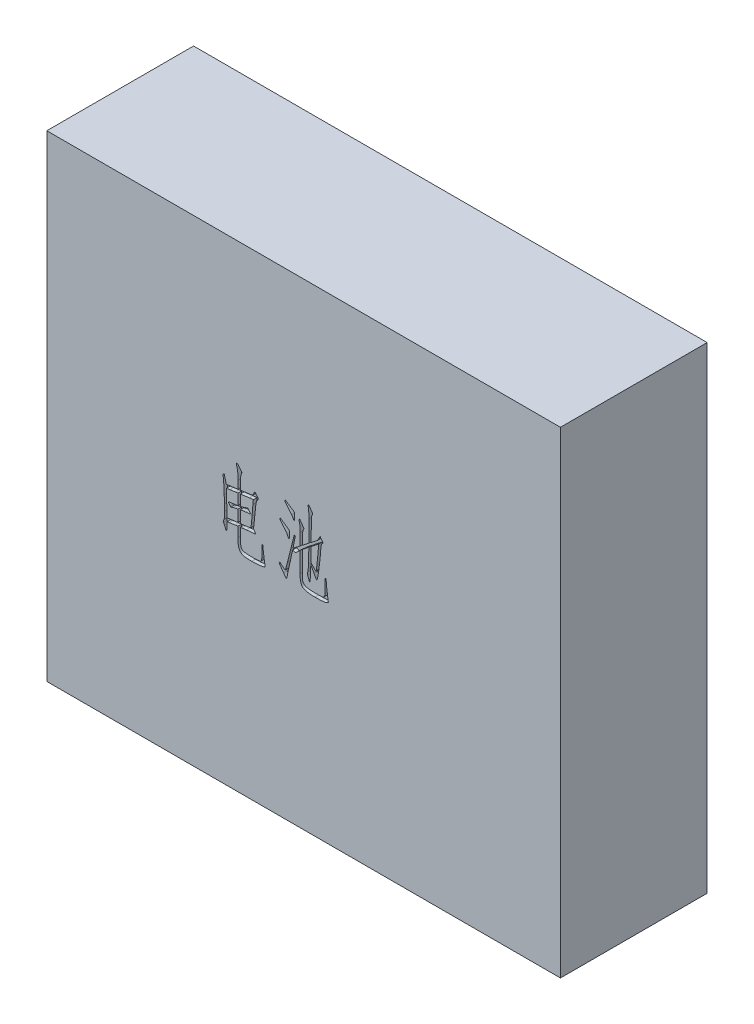
SolidWorks part; units mm, degrees
ref_plane "Front Plane" through (0, 0, 0) normal (0, 0, 1) x (1, 0, 0)
ref_plane "Top Plane" through (0, 0, 0) normal (0, 1, 0) x (1, 0, 0)
ref_plane "Right Plane" through (0, 0, 0) normal (1, 0, 0) x (0, 0, -1)
other "Configuration Table"
sketch "Sketch1" plane through (0, 0, 0) normal (0, 0, 1) x (1, 0, 0)
  line L1 (0, 0) -> (-70, 0)
  line L2 (0, 0) -> (0, 65)
  line L3 (0, 65) -> (-70, 65)
  line L4 (-70, 0) -> (-70, 65)
  dimension "D1" = 70
  dimension "D2" = 65
extrude "Boss-Extrude1" add sketch "Sketch1" along normal blind 20
sketch "Sketch2" plane through (0, 0, 20) normal (0, 0, 1) x (1, 0, 0)
  line L0 (-47.4818, 29.6161) -> (-11.9284, 29.6161) construction
  text T0 "电池" font "汉仪长仿宋体" height 8
extrude "Cut-Extrude1" cut sketch "Sketch2" against normal blind 0.5
